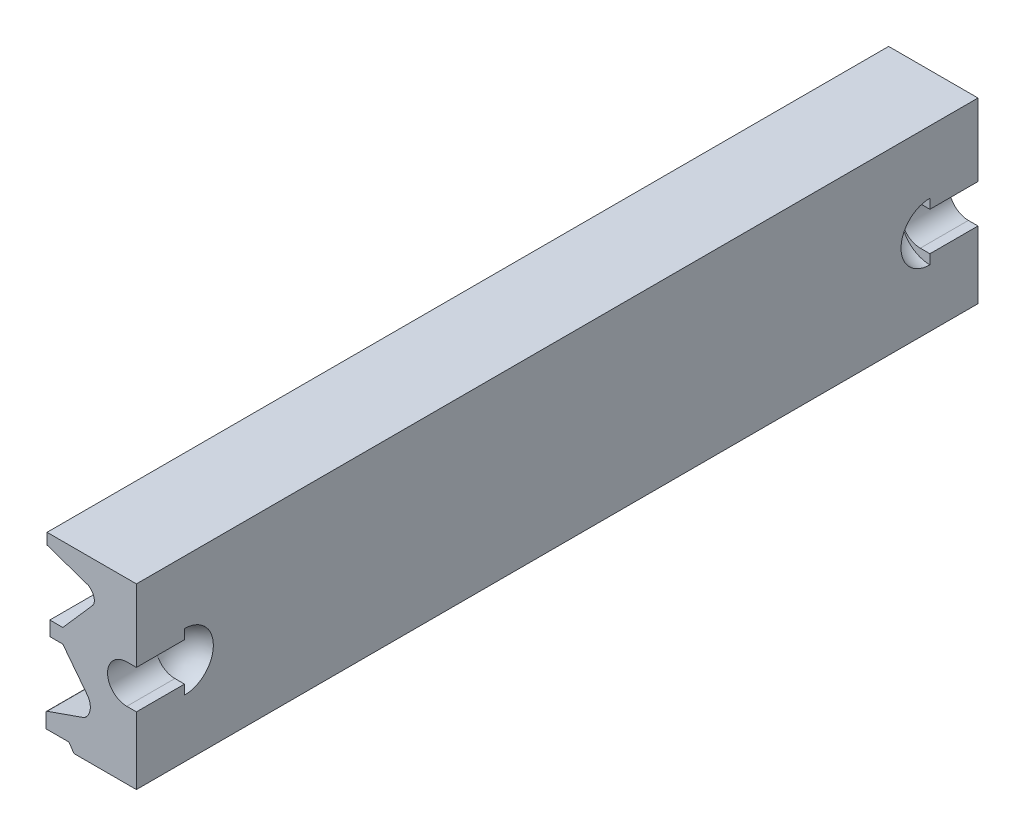
from build123d import *

# Parameters (mm, degrees)
EXTRUDE_1_DEPTH     = 1750
CUT_EXTRUDE_3_DEPTH = 100
CUT_REVOLVE_1_ANGLE = 90


with BuildPart() as part:
    # 草图1 → 凸台-拉伸1 (new body)
    with BuildSketch(Plane.XY):
        with BuildLine():
            Line((-130, -144.638291086), (0, -144.638291086))
            Line((0, -144.638291086), (0, -4.188946248))
            Line((0, -4.188946248), (0, 75.811053752))
            Line((0, 75.811053752), (0, 185.69710624))
            Line((0, 185.69710624), (0, 225.814837569))
            Line((0, 225.814837569), (-108.083873316, 225.814837569))
            Line((-108.083873316, 225.814837569), (-185.80387332, 225.814837569))
            Line((-185.80387332, 225.814837569), (-185.80387332, 202.814837569))
            Line((-185.80387332, 202.814837569), (-100.01423666, 173.289453092))
            add(Edge.make_bspline(
                [(-100.01423666, 173.289453092), (-89.242307137, 167.173453817), (-82.491572572, 150.19537082), (-92.192076155, 140.122990005)],
                knots=[0, 0, 0, 0, 1, 1, 1, 1], degree=3))
            Line((-92.192076155, 140.122990005), (-153.01423666, 70.814837569))
            Line((-153.01423666, 70.814837569), (-180.01423666, 70.814837569))
            Line((-180.01423666, 70.814837569), (-180.01423666, 40.814837569))
            Line((-180.01423666, 40.814837569), (-153.01423666, 40.814837569))
            Line((-153.01423666, 40.814837569), (-102.31538594, -24.896770131))
            ThreePointArc((-102.31538594, -24.896770131), (-95.998763417, -48.223878967), (-108.02699364, -69.185162431))
            Line((-108.02699364, -69.185162431), (-185.80387332, -96.42399324))
            add(Edge.make_bspline(
                [(-187.99699364, -99.18894625), (-187.738237709, -97.242367883), (-185.80387332, -96.42399324)],
                knots=[0, 0, 0, 1, 1, 1], degree=2))
            Line((-187.99699364, -99.18894625), (-187.99699364, -129.188946248))
            Line((-187.99699364, -129.188946248), (-140.299563226, -129.188946248))
            Line((-140.299563226, -129.188946248), (-130, -144.638291086))
        make_face()
    extrude(amount=-EXTRUDE_1_DEPTH)

    # 草图3 → 切除-拉伸3 (cut)
    with BuildSketch(Plane.XY):
        with BuildLine():
            Line((0, -4.638291086), (-20, -4.638291086))
            ThreePointArc((-20, -4.638291086), (-60, 35.361708914), (-20, 75.361708914))
            Line((-20, 75.361708914), (0, 75.361708914))
            Line((0, 75.361708914), (0, -4.638291086))
        make_face()
    cut_extrude_3 = extrude(amount=-CUT_EXTRUDE_3_DEPTH, mode=Mode.SUBTRACT)

    # 草图5 → 切除-旋转1 (revolve, cut)
    with BuildSketch(Plane(origin=(0, 0, 0), x_dir=(0, 0, -1), z_dir=(1, 0, 0))):
        with BuildLine():
            Line((100, 95.361708914), (100, -24.638291086))
            ThreePointArc((100, -24.638291086), (160, 35.361708914), (100, 95.361708914))
        make_face()
    cut_revolve_1 = revolve(axis=Axis((0, 95.361708914, -100), (0, 1, 0)), revolution_arc=CUT_REVOLVE_1_ANGLE, mode=Mode.SUBTRACT)

    # 镜向1: 切除-拉伸3, 切除-旋转1 across plane
    add(cut_extrude_3.mirror(Plane.XY.offset(-875)), mode=Mode.SUBTRACT)
    add(cut_revolve_1.mirror(Plane.XY.offset(-875)), mode=Mode.SUBTRACT)


solid = part.part
